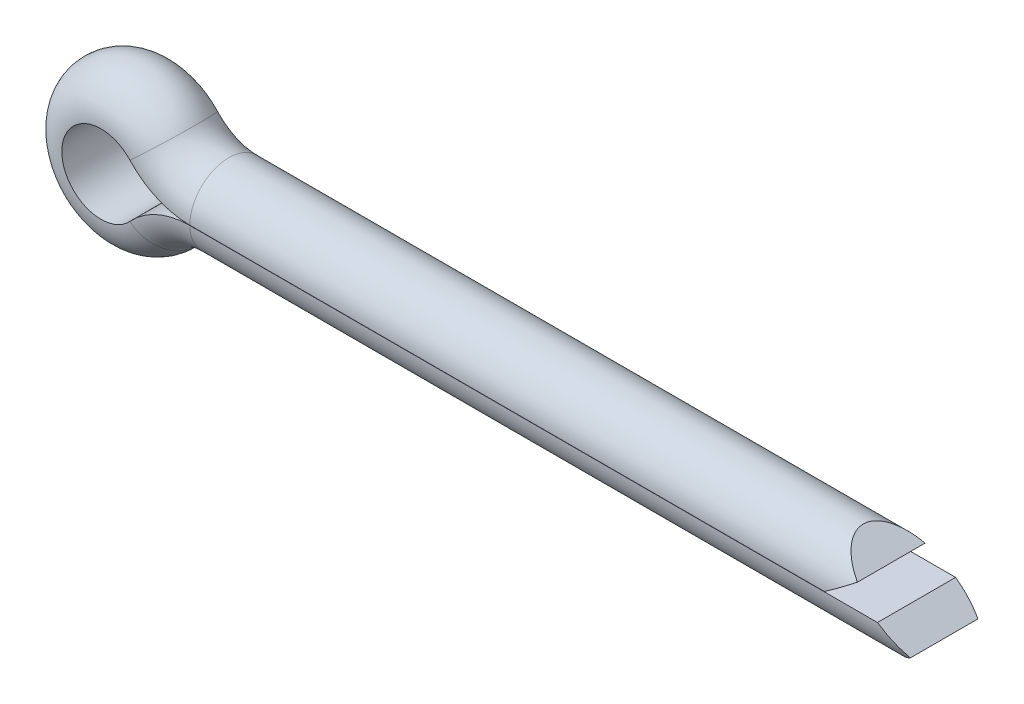
SolidWorks part; units mm, degrees
material "Q235"
ref_plane "Front Plane" through (0, 0, 0) normal (0, 0, 1) x (1, 0, 0)
ref_plane "Top Plane" through (0, 0, 0) normal (0, 1, 0) x (1, 0, 0)
ref_plane "Right Plane" through (0, 0, 0) normal (1, 0, 0) x (0, 0, -1)
sketch "Dimension sketch" plane through (0, 0, 0) normal (0, 0, 1) x (1, 0, 0)
  line L0 (56.7, 2.95) -> (6.7, 2.95)
  line L1 (6.7, -2.95) -> (60.7, -2.95)
  line L2 (6.7, 0) -> (27.3859, 0) construction
  line L3 (6.7, 0) -> (6.7, -0.0723) construction
  line L4 (-5.9, 0) -> (-5.9, 18.8979) construction
  arc A0 (6.7, 2.95) -> (4.3519, 3.9839) centre (6.7, 6.1335) cw
  arc A1 (4.3519, 3.9839) -> (4.3519, -3.9839) centre (0, 0) ccw
  arc A2 (4.3519, -3.9839) -> (6.7, -2.95) centre (6.7, -6.1335) cw
  dimension "c" = 11.8
  dimension "d1" = 5.9
  dimension "b" = 12.6
  dimension "l" = 50
  dimension "a" = 4
ref_plane "Plane1" through (56.7, 2.95, 0) normal (-1, 0, 0) x (0, 0, 1)
sketch "Sketch2" plane through (56.7, 2.95, 0) normal (-1, 0, 0) x (0, 0, 1)
  line L0 (0, -8.85) -> (0, 2.95) construction
  line L1 (-2.95, -2.94) -> (2.95, -2.94)
  arc A0 (2.95, -2.94) -> (-2.95, -2.94) centre (0, -2.95) ccw
  dimension "d" = 5.9
  dimension "D1" = 0.01
sweep "Sweep2" add profiles "Sketch2" path "Dimension sketch"
sketch "Sketch3" plane through (0, 0, 0) normal (0, 0, 1) x (1, 0, 0)
  line L0 (6.7, 0) -> (6.7, 16.2682) construction
  line L1 (6.7, 0) -> (37.4999, 0) construction
  line L2 (60.7, -2.95) -> (60.7, -0.01) construction
  line L3 (56.7, 1.47) -> (54.597, 2.95)
  line L4 (56.7, 2.95) -> (6.7, 2.95) construction
  line L5 (6.7, -2.95) -> (60.7, -2.95) construction
  line L6 (56.7, 1.47) -> (54.59, 0)
  line L7 (60.7, -1.48) -> (58.597, 0)
  line L9 (60.7, -1.48) -> (58.59, -2.95)
  line L10 (58.597, 0) -> (54.59, 0)
  line L11 (54.597, 2.95) -> (60.71, 2.95)
  line L12 (60.71, 2.95) -> (60.71, -2.95)
  line L13 (60.71, -2.95) -> (58.59, -2.95)
  line L14 (56.7, 2.95) -> (56.7, 0.01) construction
  dimension "D1" = 0.01
  dimension "D3" = 70
  dimension "D4" = 70
extrude "Cut-Extrude1" cut sketch "Sketch3" against normal through all and the other way through all
